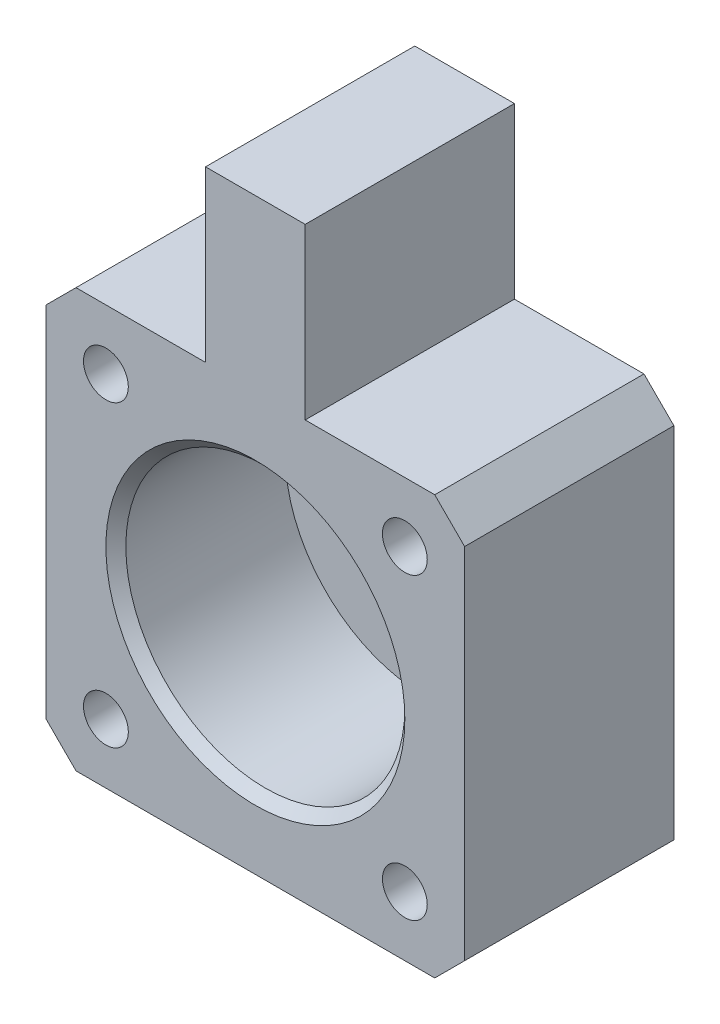
SolidWorks part; units mm, degrees
material "6063-T6"
ref_plane "前视" through (0, 0, 0) normal (0, 0, 1) x (1, 0, 0)
ref_plane "上视" through (0, 0, 0) normal (0, 1, 0) x (1, 0, 0)
ref_plane "右视" through (0, 0, 0) normal (1, 0, 0) x (0, 0, -1)
sketch "草图1" plane through (0, 0, 0) normal (0, 0, 1) x (1, 0, 0)
  line L1 (-21, 2.25) -> (21, 2.25)
  line L2 (-21, 2.25) -> (-21, 44.25)
  line L3 (-21, 44.25) -> (21, 44.25)
  line L4 (21, 2.25) -> (21, 44.25)
  line L5 (-21, 2.25) -> (21, 44.25) construction
  line L6 (-21, 44.25) -> (21, 2.25) construction
  point P0 (0, 23.25)
  dimension "D1" = 42
  dimension "D2" = 42
extrude "凸台-拉伸1" add sketch "草图1" along normal blind 12
sketch "草图2" plane through (0, 0, 12) normal (0, 0, 1) x (1, 0, 0)
  line L0 (0, 44.25) -> (0, 23.25) construction
  line L1 (21, 44.25) -> (-21, 44.25) construction
  line L2 (0, 23.25) -> (21, 23.25) construction
  line L3 (21, 2.25) -> (21, 44.25) construction
  circle A0 centre (0, 23.25) radius 14
  dimension "D1" = 28
extrude "切除-拉伸1" cut sketch "草图2" against normal blind 8
sketch "草图3" plane through (0, 0, 4) normal (0, 0, 1) x (1, 0, 0)
  circle A0 centre (0, 23.25) radius 8
  dimension "D1" = 16
extrude "切除-拉伸2" cut sketch "草图3" against normal through all
chamfer "倒角1" distance 3 angle 45 4 edges at (21, 2.25, 6) (-21, 2.25, 6) (-21, 44.25, 6) (21, 44.25, 6)
hole_wizard "打孔尺寸根据内六角圆柱头螺钉的类型2" positions "草图9" profile "草图8" counterbore size "M4" standard "Gb" end condition through all
sketch "草图9" plane through (0, 0, 0) normal (0, 0, -1) x (-1, 0, 0)
  point P0 (-15, 38.25)
  point P3 (15, 38.25)
  point P6 (15, 8.25)
  point P9 (-15, 8.25)
sketch "草图8" plane through (15, 38.25, 0) normal (1, 0, 0) x (0, 1, 0)
  line L0 (0, 0) -> (0, 12)
  line L1 (0, 12) -> (2.25, 12)
  line L3 (2.25, 12) -> (2.25, 4.6)
  line L4 (2.25, 4.6) -> (4, 4.6)
  line L5 (4, 4.6) -> (4, 0)
  line L7 (4, 0) -> (0, 0)
  line L11 (0, -6.35) -> (0, 107.95) construction
  dimension "通孔孔直径" = 4.5
  dimension "通孔孔深度" = 12
  dimension "柱形沉头孔直径" = 8
  dimension "柱形沉头孔深度" = 4.6
sketch "草图10" plane through (0, 0, 12) normal (0, 0, 1) x (1, 0, 0)
  line L8 (-18, 2.25) -> (18, 2.25)
  line L9 (18, 2.25) -> (21, 5.25)
  line L10 (21, 5.25) -> (21, 41.25)
  line L11 (21, 41.25) -> (18, 44.25)
  line L12 (18, 44.25) -> (-18, 44.25)
  line L13 (-18, 44.25) -> (-21, 41.25)
  line L14 (-21, 41.25) -> (-21, 5.25)
  line L15 (-21, 5.25) -> (-18, 2.25)
  line L16 (-18, 2.25) -> (18, 2.25)
  line L17 (18, 2.25) -> (21, 5.25)
  line L18 (21, 5.25) -> (21, 41.25)
  line L19 (21, 41.25) -> (18, 44.25)
  line L20 (18, 44.25) -> (-18, 44.25)
  line L21 (-18, 44.25) -> (-21, 41.25)
  line L22 (-21, 41.25) -> (-21, 5.25)
  line L23 (-21, 5.25) -> (-18, 2.25)
  circle A0 centre (-15, 38.25) radius 2.25 construction
  circle A1 centre (0, 23.25) radius 14 construction
  circle A2 centre (15, 38.25) radius 2.25 construction
  circle A3 centre (15, 8.25) radius 2.25 construction
  circle A4 centre (-15, 8.25) radius 2.25 construction
  circle A5 centre (-15, 38.25) radius 2.25
  circle A6 centre (0, 23.25) radius 14
  circle A7 centre (15, 38.25) radius 2.25
  circle A8 centre (15, 8.25) radius 2.25
  circle A9 centre (-15, 8.25) radius 2.25
  dimension "D1" = 0
extrude "凸台-拉伸2" add sketch "草图10" along normal blind 9
sketch "草图11" plane through (0, 0, 0) normal (0, 0, -1) x (-1, 0, 0)
  line L0 (-5, 44.25) -> (-5, 61.25)
  line L1 (-18, 44.25) -> (18, 44.25) construction
  line L2 (-5, 61.25) -> (5, 61.25)
  line L3 (5, 61.25) -> (5, 44.25)
  line L4 (5, 44.25) -> (-5, 44.25)
  line L5 (-21, 5.25) -> (-21, 41.25) construction
  dimension "D1" = 10
  dimension "D2" = 16
extrude "凸台-拉伸3" add sketch "草图11" against normal up to vertex (21 mm away)
hole_wizard "M3 螺纹孔1" positions "草图13" profile "草图12" tap size "M3" standard "Iso"
sketch "草图13" plane through (0, 0, 0) normal (0, 0, -1) x (-1, 0, 0)
  line L0 (-18, 44.25) -> (-5, 44.25) construction
  line L1 (-5, 61.25) -> (-5, 44.25) construction
  point P0 (0, 57.75)
  point P2 (0, 39.25)
  dimension "D1" = 13.5
  dimension "D2" = 18.5
  dimension "D3" = 5
sketch "草图12" plane through (0, 57.75, 0) normal (1, 0, 0) x (0, 1, 0)
  line L0 (0, 0) -> (0, 7.7511)
  line L1 (0, 7.7511) -> (1.25, 7)
  line L2 (1.25, 7) -> (1.25, 0)
  line L5 (1.25, 0) -> (0, 0)
  line L10 (0, 7.7511) -> (-1.25, 7) construction
  line L11 (0, -6.35) -> (0, 107.95) construction
  dimension "螺纹孔钻头直径" = 2.5
  dimension "螺纹孔钻头深度" = 7
  dimension "导头角度" = 118
cosmetic thread "孔螺蚊线1" parameters "D1"=6, "D2"=3
cosmetic thread "孔螺蚊线2" parameters "D1"=6, "D2"=3
chamfer "倒角2" distance 1 angle 45 1 edges at (14, 23.25, 21)
